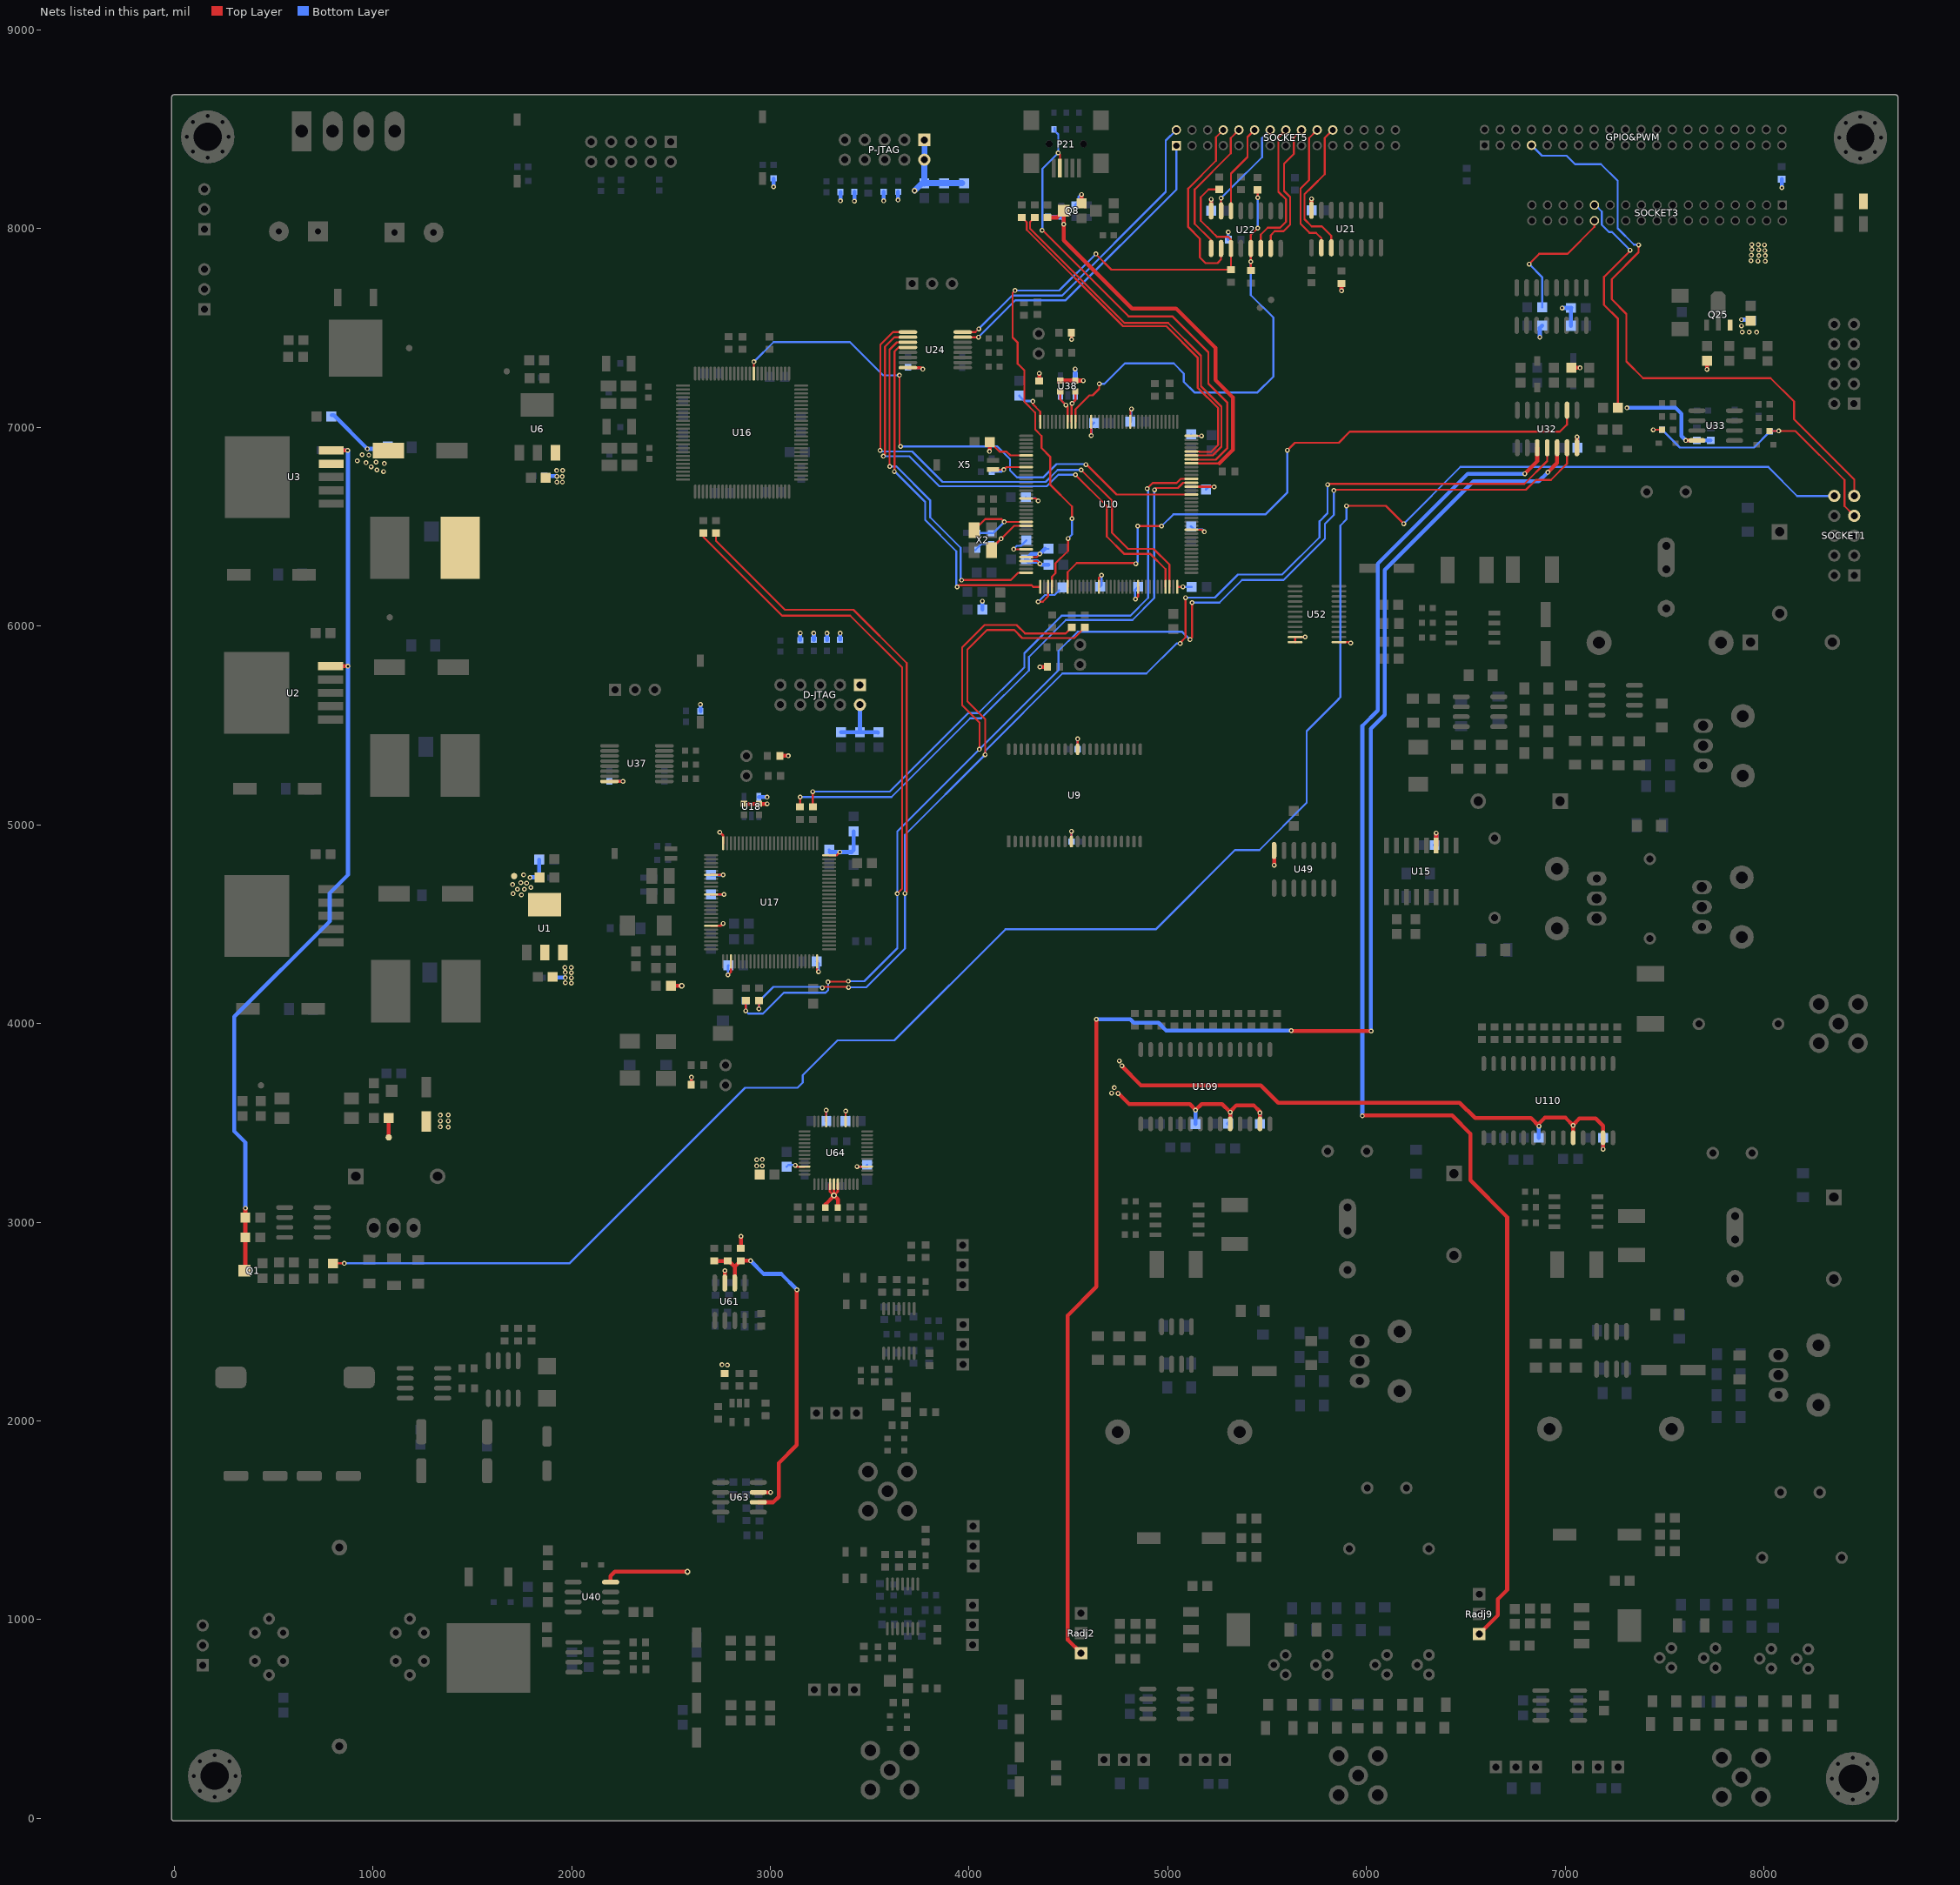
[diagram p0: the nets of this part, all layers, seen from the top]
# Altium PCB MISC82309.PcbDoc (part 12 of 14)
Units mil, origin at the board's own origin, x right, y up, seen from the top; angles counter-clockwise.
Board outline 8687.03 x 8687.86 mil, 4 copper layers (Top Layer, GND, POWER, Bottom Layer); 747 components, 583 nets, 2530 pads, 1834 vias.

## Via types
v1: diameter 24, hole 12, Top Layer to Bottom Layer, 1799 vias
v2: diameter 30, hole 15, Top Layer to Bottom Layer, 26 vias
v3: diameter 40, hole 20, Top Layer to Bottom Layer, 9 vias

## Nets (pads, with @x,y where several pads share a name; then routed paths per layer and width w, separated by ;. In a path a pad name is that pad's centre, name@x,y a point inside that pad or via, vN(x,y) a via of type N, cw(c..) or ccw(c..) an arc to the next point about the centre after c; other vN are vias at no path point) (continued)
P_OSC32_OUT: C99.2 U10.9 X5.4 | length 237.1
  Top Layer w10: X5.4@4121,6787.38 v1@4175.38,6787.38 ; v1(4175,6787) v1@4175.38,6787.38 ; U10.9@4287.65,6800.01 4189.01,6800.01 4176.38,6787.38 v1@4175.38,6787.38
  Bottom Layer w10: C99.2@4114.5,6777 4165,6777 v1(4175,6787)
P_OSC_IN: C40.2 R66.1 U10.23 X2.1 | length 459.3
  Top Layer w10: X2.1@4026,6483 4081,6538 4164,6538 v1(4177.58,6524.42) U10.23@4287.65,6524.42
  Bottom Layer w10: C40.2@4032.5,6469 4109.5,6469 R66.1@4111,6467.5 4120.67,6467.5 v1(4177.58,6524.42)
P_OSC_OUT: C41.2 R66.2 U10.24 X2.3 | length 381.6
  Top Layer w10: X2.3@4112.61,6383 4112.61,6390.61 4226.73,6504.73 U10.24@4287.65,6504.73
  Bottom Layer w10: C41.2@4032.5,6383 4062,6412.5 R66.2@4111,6412.5 4134.5,6412.5 v1(4161,6439)
P_RS232_RXD: SOCKET5.2 U24.8 | length 1648.1
  Top Layer w10: U24.8@3967.8,7479.57 4032.57,7479.57 v1(4049,7496)
  Bottom Layer w10: v1(4049,7496) 4217,7664 4469,7664 4990,8185 4990,8443.74 SOCKET5.2@5043,8496.74
P_RS232_TXD: SOCKET5.1 U24.7 | length 1604
  Top Layer w10: U24.7@3967.8,7453.98 v1(4048,7454)
  Bottom Layer w10: v1(4048,7454) 4234,7640 4486,7640 5043,8197 SOCKET5.1@5043,8418
P_SCL: R208.2 U10.136 U38.1 | length 206.2
  Top Layer w10: U10.136@4515.99,7028.35 4515.99,7069 4515.99,7117.99 v1(4519,7121) 4535,7137 R208.2@4535,7180.5
  Bottom Layer w10: v1(4519,7121) 4534.4,7136.4 U38.1@4534.4,7160.76
P_SDA: R209.2 U10.137 U38.3 | length 227.2
  Top Layer w10: R209.2@4459,7180.5 4459,7141 4487,7113 v1(4487.35,7112.65) 4496.31,7103.69 4496.31,7089 U10.137@4496.31,7028.35
  Bottom Layer w10: U38.3@4459.6,7160.76 4459.6,7140.4 v1(4487.35,7112.65)
P_USART2_RX: U10.37 U24.12 | length 1814.6
  Top Layer w10: v1@3625,6779 3625,7382 3645.8,7402.8 U24.12@3692.2,7402.8 ; v1@3940,6198 3947.5,6205.5 4314.5,6205.5 4322.35,6197.65 U10.37@4358.51,6197.65
  Bottom Layer w10: v1@3626,6778 3779,6625 3779,6534 3936,6377 3936,6204 v1@3942,6198
  other v1: 3940,6197 3624,6778
P_USART2_TX: U10.36 U24.11 | length 1774.7
  Top Layer w10: v1@3600,6804 3600,7391 3637.39,7428.39 U24.11@3692.2,7428.39 ; v1@3963,6232 4210,6232 4246.51,6268.51 U10.36@4287.65,6268.51
  Bottom Layer w10: v1(3601,6803) 3635,6803 3806,6632 ; 3805,6631 3805,6547 3958,6394 3958,6237 v1@3963,6232
  other v1: 3963,6231
P_USART3_RX: U10.70 U24.9 | length 2647.5
  Top Layer w10: v1@3554,6884 3554,7416 3617.57,7479.57 U24.9@3692.2,7479.57 ; v1(4564,6786) 4719,6631 4719,6470 4800,6389 4929,6389 5008.12,6309.88 U10.70@5008.12,6197.65
  Bottom Layer w10: v1(3552,6884) 3558,6878 3558.06,6878 3559.06,6879 3714,6879 3867,6726 4386,6726 4446,6786 v1(4564,6786)
P_USART3_TX: U10.69 U24.10 | length 2577.3
  Top Layer w10: v1(3569,6855) 3577,6863 3577,7406 3624.98,7453.98 U24.10@3692.2,7453.98 ; v1@4535,6756 v1(4535,6762) 4693,6604 4693,6450.72 4779.72,6364 4911.43,6364 4988.43,6287 U10.69@4988.43,6197.65
  Bottom Layer w10: v1(3569,6855) 3699,6855 3850,6704 4391,6704 4449,6762 v1(4535,6762)
P_VDDA: C37.2 C38.2 R276.2 U10.32 U10.33 | length 452.8
  Top Layer w10: U10.33@4287.65,6327.57 4343.43,6327.57 v1(4357,6314) ; U10.32@4287.65,6347.25 4340.25,6347.25 v1(4356,6363)
  Bottom Layer w10: v1(4356,6363) 4382,6389 C37.2@4399.5,6389 ; C38.2@4394.5,6314 C38.2@4399.5,6309
  Bottom Layer w20: C37.2@4382,6389 v1(4356,6363) 4313.5,6363 R276.2@4286.5,6336 4297.5,6325 4346,6325 v1(4357,6314) 4362,6309 C38.2@4399.5,6309
POWER-ON/OFF: GPIO&PWM.7 SOCKET1.9 | length 3090.6
  Top Layer w10: v1@7364,7918 v1(7369,7918) ; v1@7369,7916 7369,7881 7234,7746 7234,7645 7308,7571 7308,7332 7392,7248 8033,7248 8151,7130 8151,7041 8454,6738 SOCKET1.9@8454,6655
  Bottom Layer w10: GPIO&PWM.7@6830.22,8420 6883.22,8367 7007,8367 7049,8325 7180,8325 7264,8241 7264,8002 7346,7920 ; 7346,7919 v1@7366,7919 ; v1@7364,7918 v1(7369,7918)
POWER_CONTROL: R8.1 SOCKET1.10 | length 10132.2
  Top Layer w10: R8.1@799.5,2793 v1(856,2793) ; v1(5899,6605) 6097,6605 v1(6187,6515)
  Bottom Layer w10: v1(856,2793) 1989,2793 2873,3677 3137,3677 3163,3703 3163,3740 3338,3915 3624,3915 4183,4474 4939,4474 5338,4873 5461,4873 5699,5111 5699,5472 5860.5,5633.5 ; 5860,5634 5868,5642 5868,6506 5899,6537 v1(5899,6605) ; v1@6189,6517 6473,6801 8022,6801 ; 8022,6800 8167,6655 SOCKET1.10@8354,6655 SOCKET1.10@8349.5,6659.5
POWER_ENABLE: Q1.3 R7.1 R399.2 R555.2 U2.5 U3.5 | length 4637.2
  Top Layer w20: Q1.3@354,2756 358.5,2760.5 R399.2@358.5,2924 R7.1@358.5,3024 v1(358.5,3070.5) ; U2.5@787.22,5797.86 v1(874.86,5797.86) ; U3.5@790.22,6883.86 v1(872.86,6883.86)
  Bottom Layer w20: v1(358.5,3070.5) 358.5,3402.5 303,3458 303,4034 783,4514 783,4656 875,4748 875,6882 v1@873,6884 ; R555.2@797,6885 798.14,6883.86 v1(872.86,6883.86)
PRE-CH_A: R345.2 R349.2 R515.2 R565.1 U32.13 | length 9740.3
  Top Layer w10: R345.2@2663,6468.5 2663,6449 3059,6053 3402,6053 3663,5792 3663,4678 v1@3638.5,4653.5 ; v1@2877,4065 R515.2@2877,4115.5 ; v1@3292,4211 v1@3390,4211 ; v1(4052,5380) 4053,5381 4053,5514 3965,5602 3965,5893 4078,6006 4239,6006 4282.21,5962.79 4486.28,5962.79 R349.2@4517,5993.5 ; 5122,5942 v1(5122,6118) ; v1(5836,6682) 5840,6686 6802,6686 6852,6736 6928,6736 7009,6817 U32.13@7009,6897.51
  Bottom Layer w10: v1(2876,4064) 2890,4050 2963,4050 3068,4155 3278,4155 3291,4168 v1@3291,4208 ; v1@2876,4067 R565.1@2876,4115.5 ; v1(3392,4213) 3473,4213 3639,4379 v1(3639,4653) 3639,4967 v1(4052,5380) 4450,5778 4450,5875 4546,5971 5073,5971 v1(5112,5932) ; v1(5122,6118) 5260,6118 5374,6232 5583,6232 5791,6440 5791,6514 5836,6559 v1(5836,6682)
  other v1: 3290,4209
PRE-CH_B: R346.2 R348.2 R516.2 R564.1 U32.11 | length 9489.9
  Top Layer w10: R346.2@2727,6468.5 2727,6429 3074,6082 3418,6082 3686,5814 v1@3686,4663 ; v1@2943,4067 R516.2@2943,4115.5 ; v1@3267,4185 v1@3394,4185 ; v1(4081,5353) 4081,5532 3992,5621 3992,5882 4090,5980 4228,5980 4268,5940 4529.5,5940 R348.2@4583,5993.5 ; v1@5062,5915.94 5089,5942.94 v1(5089,6143) ; v1(5804,6712) 5808,6716 6794,6716 6909,6831 U32.11@6909,6897.51
  Bottom Layer w10: v1@2940,4071 v1@2940,4072 ; v1@2943,4070 2943,4112 3016,4185 v1@3257,4185 ; v1(2943,4074) 2943,4067 v1@2944.5,4068.5 ; v1(3394,4182) 3483,4182 3678,4377 v1(3678,4655) 3678,4950 v1(4081,5353) 4081,5372 4470,5761 4892,5761 5044,5913 v1(5062,5913) ; v1(5089,6143) 5237,6143 5353,6259 5575,6259 5763,6447 5763,6527 5804,6568 v1(5804,6712) 5806,6710 v1@5806,6712
  other v1: 3262,4180
PRE-CHARGE_A: Radj2.1 U32.12 | length 8198
  Top Layer w20: Radj2.1@4564,832 4497,899 4497,2531 4641,2675 v1(4641,4022) ; v1(5621,3965) 5624,3962 v1(6023,3962) ; v1(6912,6774) 6959,6821 U32.12@6959,6897.51
  Bottom Layer w20: v1(4641,4022) 4811,4022 4829,4004 4953,4004 4992,3965 v1(5621,3965) ; v1@6021,3965 6022,3966 6022,5484 6091,5553 6091,6282 6538,6729 6867,6729 v1(6912,6774)
PRE-CHARGE_B: Radj9.1 U32.10 | length 7127.3
  Top Layer w20: v1@5980,3537 6431,3537 6523,3445 6523,3211 6708,3026 6708,1150 6661,1103 6661,1022 Radj9.1@6567,928 ; v1(6797,6767) 6859,6829 U32.10@6859,6897.51
  Bottom Layer w20: v1(5979,3536) 5979,5498 6057,5576 6057,6314 6510,6767 v1(6797,6767)
PRINT-RST: U10.93 U16.85 | length 2907.2
  Top Layer w10: U16.85@2917.06,7271.24 v1(2917.06,7329.94) ; v1@3650,6910 v1(3650,7262) ; v1(4588,6813) 4591,6813 4742,6662 5118.14,6662 U10.93@5118.35,6662.21
  Bottom Layer w10: v1(2917.06,7329.94) 3016.11,7429 3401,7429 3568,7262 v1(3650,7262) ; v1(3656,6904) 4143,6904 4206,6841 4206,6784 4242,6748 4373,6748 4440.38,6815.38 4585.62,6815.38 v1(4588,6813) v1@4589,6812
PRODUCT-S: U10.44 U32.2 | length 3194.3
  Top Layer w10: U10.44@4496.31,6197.65 4496.31,6271.31 4542,6317 v1@4836,6317 ; v1(4848,6503) v1(4969,6503) ; v1(5602,6885) 5639.91,6922.91 5860.91,6922.91 5916,6978 6973,6978 7009,7014 U32.2@7009,7086.49
  Bottom Layer w10: v1(4839,6314) 4848,6323 v1(4848,6503) ; v1(4969,6503) 5028,6562 5491,6562 5602,6673 v1(5602,6885)
PRODUCT_SENSOR_: R493.1 SOCKET3.25 | length 1192.5
  Top Layer w10: R493.1@7265.5,7098 7265.5,7546.5 7195,7617 7195,7757 7326,7888 v1(7326,7892)
  Bottom Layer w10: SOCKET3.25@7147.12,8119 SOCKET3.25@7153.06,8113.06 ; SOCKET3.25@7155,8115 7184,8086 7184,8019 7220,7983 7235,7983 v1(7326,7892) v1@7326,7888
REFINA: C506.1 C507.1 U64.5 U64.6 U64.7 | length 330.6
  Top Layer w12: U64.5@3300.47,3191.52 3300.47,3154.53 v2(3320,3135) ; U64.6@3320.16,3191.52 3320.16,3135.16 3339.84,3154.84 U64.7@3339.84,3191.52
  Top Layer w20: C506.1@3277,3075.95 3277,3077.5 C506.1@3278,3078.5 ; C506.1@3278,3076 C506.1@3278,3078.5 ; C507.1@3340,3077.5 3340,3115 3320.16,3134.84 3320.08,3134.92 v2(3320,3135) 3320,3132.41 3278,3090.41 C506.1@3278,3078.5
SENSOR_DECTET: R155.1 SOCKET3.26 | length 681.9
  Top Layer w10: v1(6818,7822) 6869,7873 7011,7873 7147.12,8009.12 SOCKET3.26@7147.12,8040.26
  Bottom Layer w10: v1(6818,7822) 6883.5,7756.5 R155.1@6883.5,7605
SENSOR_DRV: C163.2 C363.2 R175.1 R375.1 SOCKET1.7 | length 1426.9
  Top Layer w10: v1(7443,6988) R175.1@7487.5,6988 ; R375.1@8027.5,6982 v1(8074,6982) 8158,6982 8405,6735 8405,6604 SOCKET1.7@8454,6555
  Bottom Layer w10: v1(7443,6988) C163.2@7487.5,6988 7576.5,6899 7949.5,6899 C363.2@8029.5,6979 8032.5,6982 v1(8074,6982)
SPI2_CS: R101.1 R405.2 U10.40 U22.3 | length 3442.1
  Top Layer w10: v1(4231,7689) 4219,7677 4219,7452 4245,7426 4245,7320 4278,7287 4278,7264 4278,7129 4332,7075 ; 4333,7075 4333,6989 4365,6957 4365,6896 4408,6853 4408,6712 4518,6602 v1(4518,6541) ; U10.40@4417.57,6197.65 4417.57,6248.57 4435,6266 4435,6316 4498,6379 v1(4498,6441) ; v1@4636,7874 4716.5,7793.5 R405.2@5313.5,7793.5 ; 5224,7981 5225,7981 5246.5,7959.5 5303.5,7959.5 5318,7945 U22.3@5318,7900.51 5318,7794 R405.2@5319,7793 ; 5224.5,7981.5 5166,8040 5166,8158 5205.5,8197.5 R101.1@5258,8197.5 R101.1@5269,8197.5 ; R405.2@5314,7794 R405.2@5313.5,7793.5 ; R405.2@5318,7793.5 R405.2@5313.5,7793.5
  Bottom Layer w10: v1(4231,7689) 4454,7689 v1(4638,7873) ; v1(4498,6441) 4518,6461 v1(4518,6541)
SPI2_CS_N: SOCKET5.10 U22.1 | length 723
  Top Layer w10: U22.1@5218,7900.51 5218,7942 5135,8025 5135,8197 5317,8379 5317,8455.78 SOCKET5.10@5357.96,8496.74
SPI2_CS_P: SOCKET5.8 U22.2 | length 919.7
  Top Layer w10: U22.2@5268,7900.51 5268,7845 5250,7827 5190,7827 5162,7855 5162,7949 5103,8008 5103,8202 5243,8342 5243,8460.52 SOCKET5.8@5279.22,8496.74
SPI2_MISO_N: SOCKET5.22 U21.3 | length 738.3
  Top Layer w10: 5725,8210 5688,8173 5688,8048 5724,8012 5775,8012 5823,7964 U21.3@5823,7903.51 ; 5725.5,8209.5 5790,8274 5790,8456.34 SOCKET5.22@5830.4,8496.74
SPI2_MISO_P: SOCKET5.20 U21.2 | length 689.7
  Top Layer w10: 5713,7979 5746,7979 5773,7952 U21.2@5773,7903.51 ; 5713,7980 5668,8025 5668,8202 5711,8245 5711,8456.08 SOCKET5.20@5751.66,8496.74
SPI2_MOSI: R103.1 R408.2 U10.135 U22.5 | length 2336.5
  Top Layer w10: U10.135@4535.68,7028.35 4535.68,7090.68 4606,7161 4622,7161 4655,7194 v1(4655,7219) ; v1@5417,7836 5418,7835 R408.2@5418,7789.5 ; v1(5418,7834) U22.5@5418,7900.51 5418,7968 v1(5453,8003) ; R103.1@5448,8194.5 5453,8189.5 v1(5453,8156)
  Bottom Layer w10: v1(4655,7219) 4681,7219 4784,7322 5030,7322 5081,7271 5081,7229 5134,7176 5452,7176 5532,7256 5532,7552 5418,7666 v1(5418,7834) ; v1(5453,8003) v1(5453,8156)
SPI2_MOSI_N: SOCKET5.18 U22.7 | length 712.4
  Top Layer w10: U22.7@5518,7900.51 5518,7967 5538,7987 5583,7987 5616,8020 5616,8159 5585,8190 5585,8327 5634,8376 5634,8457.82 SOCKET5.18@5672.92,8496.74
SPI2_MOSI_P: SOCKET5.16 U22.6 | length 716.3
  Top Layer w10: U22.6@5468,7900.51 5468,7970 5503,8005 5565,8005 5595,8035 5595,8148 5557,8186 5557,8459.56 SOCKET5.16@5594.18,8496.74
SPI2_SCK_N: SOCKET5.14 U22.15 | length 509.7
  Top Layer w10: U22.15@5268,8089.49 v1(5268,8154)
  Bottom Layer w10: v1(5268,8154) 5321.5,8207.5 5474,8360 5474,8455.3 SOCKET5.14@5515.44,8496.74
SPI2_SCK_P: SOCKET5.12 U22.14 | length 456.4
  Top Layer w10: U22.14@5318,8089.49 5318,8278 5401.08,8361.08 5401.08,8461.12 SOCKET5.12@5436.7,8496.74
USART6_RX: R513.2 U10.97 | length 3003.2
  Top Layer w10: R513.2@3214,5090.5 v1(3214,5167) ; v1(4896,6692) 4924,6720 5044,6720 5064.95,6740.95 U10.97@5118.35,6740.95
  Bottom Layer w10: v1(3214,5167) 3601,5167 3996,5562 4048,5562 4278,5792 4278,5863 4466,6051 ; 4466,6052 4811,6052 4901,6142 4901,6687 v1(4896,6692)
USART6_TX: R514.2 U10.96 | length 3031.3
  Top Layer w10: R514.2@3150,5090.5 v1(3150,5140) ; v1(4933,6686) 4942,6695 5051,6695 5077.27,6721.27 U10.96@5118.35,6721.27
  Bottom Layer w10: v1(3150,5140) 3610,5140 4006,5536 4060,5536 4301,5777 4301,5845 4487,6031 4822,6031 4932,6141 4932,6685 v1(4933,6686)
USBDM: R95.2 U10.103 | length 1860.3
  Top Layer w10: R95.2@4330,8056.5 4307,8033.5 4307,8001.04 4782.04,7526 5001.41,7526 5167,7360.41 5167,7207.63 5270,7104.63 5270,6902.96 5226.1,6859.06 U10.103@5118.35,6859.06
USBDP: R96.2 U10.104 | length 1832.1
  Top Layer w10: R96.2@4266,8056.5 4290,8032.5 4290,7994 4775,7509 4994.37,7509 4994.37,7507.59 5150,7351.96 5150,7200.59 5253,7097.59 5253,6911.41 5218.49,6876.91 5160.84,6876.91 5159,6878.75 U10.104@5118.35,6878.75
USBID: ESD23.1 P21.4 U10.102 | length 2454.3
  Top Layer w10: v1(4368,7992) 4370,7992 4803,7559 5023,7559 5204,7378 5204,7220 5300,7124 5300,6896 5241.6,6837.6 5120.13,6837.6 U10.102@5118.35,6839.38 ; v1(4449,8381) 4457.5,8372.5 P21.4@4457.5,8304.95
  Bottom Layer w10: v1(4368,7992) 4369.25,7993.25 4369.25,8301.25 v1(4449,8381) 4449,8474 4430,8493 ESD23.1@4430,8506.68
VBUS: C240.2 C241.2 Q8.3 R57.2 U10.101 | length 2124.5
  Top Layer w11: U10.101@5118.35,6819.69 5260.69,6819.69
  Top Layer w20: R57.2@4394,8056.5 4442.5,8056.5 Q8.3@4476,8090 4476,7942 4820,7598 5042,7598 5240,7400 5240,7238 5327,7151 5327,6886 5260.69,6819.69
  Bottom Layer w20: C241.2@4397,8060.5 C240.2@4460.5,8060.5 ; C240.2@4465,8060.5 4477,8048.5 v1(4477,8023)
VCC: C1.2 C6.2 C10.1 C15.1 C17.1 C18.2 C19.2 C56.1 C82.2 C83.2 C151.2 C154.2 C210.2 C370.2 FB18.2 FB25.1 L3.2 Q8.2 R3.1 R5.1 R35.2 R36.2 R150.2 R156.2 R165.2 R479.2 TP3.1 U1.3 U3.4 U6.3 U15.11 U21.16 U22.16 U32.14 U33.8 U40.8 U49.14 U52.1 U61.3 U63.3 | length 2740
  Top Layer w12: U52.1@5861.24,5919.25 5915.75,5919.25 v1(5920,5915)
  Top Layer w20: TP3.1@1080,3427 R5.1@1080,3511 ; U40.8@2196.49,1189 2196.49,1219.49 2218,1241 v2(2583,1241) ; U61.3@2771,2694.49 v1(2771,2756) ; U63.3@2939.49,1641 v1(3001,1641) ; Q8.2@4566,8127 v1(4566,8172) ; U22.16@5218,8089.49 v1(5218,8148) ; v1(5535,4797) U49.14@5535,4870.49 ; U21.16@5723,8092.49 v1(5723,8150) ; v1(5874,7688) R35.2@5874,7724.5 ; U15.11@6351,4896 v1(6351,4959) ; R165.2@7030,7299.5 v1(7074.5,7299.5) ; U32.14@7059,6874 v1(7059,6952) ; v1(7606,6934) U33.8@7662.51,6934
  Bottom Layer w15: R150.2@4535,8119.5 4552,8136.5 4552,8159 v1@4562,8169 ; R36.2@5304.5,7945 v1(5304.5,7983.5)
  Bottom Layer w20: R3.1@793,7061 803,7061 v1@971,6893 ; v1@968,6893 v1@971,6893 ; v1@972,6893 v1@971,6893 ; C15.1@1075,6890 1073,6892 v1(972,6892) v1@971,6893 ; C19.2@1863.5,6755 v1@1925,6755 ; C6.2@1922.5,4231 1965,4231 v1@1966,4232 ; C82.2@5218.5,8090 v1@5218.5,8145.5 ; C83.2@5723,8104 v1(5723,8150) ; C56.1@6342.5,4898 6351,4906.49 v1@6351,4958 ; v1(6872,7454) 6872,7500.5 R156.2@6883.5,7512 ; v1(6984,7601) C151.2@7028.5,7601 ; FB18.2@7028.61,7511 7028.61,7601.61 C151.2@7030,7603 ; C154.2@7059,6895.51 C154.2@7060.5,6897 v1@7060.5,6950.5 ; v1(7310,7098) 7555.04,7098 7584,7069.04 7584,6956 v1(7606,6934) ; v1@7610.5,6934.5 C370.2@7663,6934.5 C210.2@7732,6934.5
  other v1: 2784,2282 2757,2283 1379,3479 1339,3480 1340,3510 1380,3510 1339,3539 1380,3540 1999,4203 1969,4205 1999,4230 1968,4231 1999,4256 1968,4257 1967,4282 1998,4282 1954,6724 1926,6725 1953,6753 1926,6754 1054,6778 1925,6783 1955,6784 1021,6786 991,6802 1058,6818 966,6822 1016,6825 921,6832 980,6860 946,6862 8006,7836 7970,7837 7935,7839 8006,7864 7974,7865 7936,7867 8004,7890 7973,7894 7938,7895 8003,7918 7938,7920 7971,7920
VDD_3V3: C2.2 C7.2 C30.1 C31.1 C86.2 C87.2 C88.2 C90.2 C123.2 C124.2 C125.2 C126.2 C127.2 C128.2 C129.2 C130.2 C131.2 C132.2 C133.2 C134.2 C141.2 C142.2 C143.2 C146.2 C147.2 C148.2 C181.2 C220.2 C242.2 C243.2 C245.2 C246.2 C247.2 C248.2 C249.2 C250.2 C251.2 C252.2 C253.2 C254.2 C255.2 C282.1 C283.1 D-JTAG.1 D-JTAG.2 L21.2 P-JTAG.1 P-JTAG.2 Q25.3 R1.1 R63.1 R111.1 R112.1 R113.1 R208.1 R209.1 R235.1 R270.2 R271.2 R272.2 R273.2 R274.2 R277.1 R283.2 R404.1 R587.2 R588.2 R589.2 R590.2 R592.2 R593.2 R594.2 R596.1 R598.2 TP1.1 U1.2 U1.4 U9.11 U9.33 U10.6 U10.17 U10.30 U10.39 U10.52 U10.62 U10.72 U10.84 U10.95 U10.108 U10.121 U10.131 U10.144 U17.6 U17.11 U17.19 U17.28 U17.50 U17.75 U17.100 U18.5 U24.16 U37.16 U38.5 U52.23 U52.24 U64.15 U64.28 U64.33 U64.46 U109.24 U109.27 U110.24 U110.27 | length 9934.1
  Top Layer w10: v1(2787,4245) v1@2788.5,4246.5 ; v1@2789,4246 2802.15,4259.15 U17.28@2802.15,4312.76 ; v1(3125,3287) 3131.9,3280.1 U64.46@3172.52,3280.1 ; U17.50@3235.22,4312.76 3235.22,4268.78 v1(3243,4261) ; U64.33@3280.79,3506.48 v1(3280.79,3563.79) ; U64.28@3379.21,3506.48 v1(3379.21,3560.21) ; v1(3436.1,3280.1) U64.15@3487.48,3280.1 ; v1(4103,6879) v1@4103,6881 ; C128.2@4103,6925.5 C128.2@4103.5,6926 ; C128.2@4122,6910 4154,6878 4189,6878 4207.94,6859.06 U10.6@4287.65,6859.06 ; v1(4224.38,6386.62) U10.30@4287.65,6386.62 ; U10.17@4287.65,6642.53 4335.47,6642.53 v1(4348,6630) ; v1@4322,7132 v1(4321,7131) 4321,7117 4358.51,7079.49 U10.144@4358.51,7028.35 ; v1(4348,6123) 4371,6123 4397.88,6149.88 U10.39@4397.88,6197.65 ; U9.11@4514.96,4916 v1(4514.96,4967.96) ; U9.33@4546.46,5380.57 v1(4546.46,5432.46) ; U10.131@4614.42,7028.35 4614.42,6959.58 v1(4615,6959) ; U10.52@4653.79,6197.65 4653.79,6242.79 v1(4667,6256) ; U10.121@4811.27,7028.35 4812,7029.09 4812,7090 4810,7092 4811,7093 v1(4817,7093) ; v1(4838,6136) 4850.64,6148.64 U10.62@4850.64,6197.65 ; U10.72@5047.49,6197.65 v1(5075.65,6197.65) ; U10.84@5118.35,6485.05 5172.95,6485.05 v1(5184,6474) ; U10.108@5118.35,6957.49 v1(5169.51,6957.49)
  Top Layer w12: U17.19@2701.76,4491.89 2750.89,4491.89 v1(2763,4504) ; U17.11@2701.76,4649.37 v1(2767.63,4649.37) ; U17.6@2701.76,4747.8 v1(2762.8,4747.8) ; v1(2746,4963) 2762.78,4946.22 U17.100@2762.78,4907.24 ; U17.75@3296.24,4846.22 3333.22,4846.22 v1(3350,4863) ; U10.95@5118.35,6701.58 v1@5230.58,6701.58 ; v1@5231,6702 v1@5230.58,6701.58 ; v1(5233,6701) 5232,6701 5231.42,6701.58 v1@5230.58,6701.58 ; U52.24@5640.76,5919.25 5641,5919.49 U52.23@5641,5943 ; U52.23@5640.76,5944.84 v1(5690.84,5944.84)
  Top Layer w15: U37.16@2191.2,5218.43 v1(2258.43,5218.43) ; R272.2@2602.5,3691 v1(2602.5,3729.5)
  Top Layer w16: U24.16@3692.2,7300.43 v1@3758.57,7300.43 ; v1(4515.5,7442.5) R271.2@4515.5,7476
  Top Layer w20: R235.1@2499.5,4190 v2(2554,4190) ; R598.2@2852,2869.5 2852,2923 v1(2852,2929) ; R112.1@2868,5105.5 R111.1@2939.5,5105.5 ; R111.1@2943,5105.5 v1(2984.5,5105.5) ; R273.2@3048.5,5347 v1(3090,5347) ; C128.2@4103.5,6926 4103.5,6881.5 v1@4104,6881 ; R274.2@4353,7234 v1(4353,7272) ; v1(4357,5794) 4362,5794 4363,5795 R270.2@4393.5,5795 ; R209.1@4459,7235.5 v1(4575.5,7235.5) ; v1@4749,3651 4806,3594 5111,3594 5140,3565 5170,3595 5273,3595 v1(5314,3554) U109.24@5314,3494.99 ; v1@4767,3787 4865,3689 5468,3689 5555,3602 6469,3602 6547,3524 6828,3524 v1@6867,3485 ; v1@5315,3558 5346,3589 5432,3589 5464,3557 v1(5464,3550) U109.27@5464,3494.99 ; v1(6868,3484) v1@6867,3485 ; U110.24@7040,3424.99 v1(7040,3487) 7001,3526 6898,3526 6867,3495 v1@6867,3485 ; v1@7041,3492 7071,3522 7153,3522 7190,3485 U110.27@7190,3424.99 v1(7190,3368) ; v1(7713,7292) R283.2@7713,7335.5
  Bottom Layer w10: C86.2@3082,3279.5 3090.5,3288 v1@3122,3288 ; C252.2@3233.5,4313 3244,4302.5 v1@3244,4266 ; C254.2@3282.5,3509 v1@3282.5,3561.5 ; C243.2@3378.5,3509 v1@3378.5,3556.5 ; v1@3437,3280 3478.5,3280 C250.2@3488,3289.5 ; v1@4226,6390 4240,6404 4260.5,6404 C130.2@4289,6432.5 ; C129.2@4285.5,6649 4290.5,6644 4333,6644 v1@4345,6632 ; v1(4348,6123) 4382,6157 4431,6157 C143.2@4453,6179 ; v1@4515,4965 v1@4515.5,4964.5 ; v1(4546.46,5432.46) 4546.5,5432.41 C148.2@4546.5,5381 ; C142.2@4660.5,6198 4667,6204.5 v1(4667,6256) v1@4667,6258 ; C125.2@4811.5,7028 4817,7033.5 v1@4817,7089 ; v1@4835,6140 4835,6182.5 C134.2@4850.5,6198 ; v1(5075.65,6197.65) 5076.29,6197 C141.2@5120.5,6197 ; C124.2@5118,6964.5 5126.5,6956 v1@5170,6956
  Bottom Layer w12: C245.2@2701,4649.5 2760.5,4649.5 v1@2761,4649 ; C87.2@2701,4747.5 2759.5,4747.5 v1@2760,4748 ; v1@2788,4247 2787,4246 2787,4290.5 C251.2@2789.5,4293 ; C247.2@3296,4875.5 C247.2@3308.5,4863 ; C127.2@4253,7159.5 4279.5,7133 v1@4321,7133 ; C147.2@4515.5,4915 v1@4515.5,4964.5 ; v1@4615,6961 4615,7009.5 C126.2@4628.5,7023 ; C123.2@5117,6501.5 5132.5,6486 5174,6486 v1@5183,6477 ; C146.2@5192.5,6688 5205.5,6701 v1@5232,6701
  Bottom Layer w15: C181.2@2191,5218.5 v1@2254.5,5218.5
  Bottom Layer w16: C90.2@3693,7302.5 3695.5,7300 3758,7300 v1@3764,7294
  Bottom Layer w20: v1@1794,4736 1834,4736 1837.5,4739.5 R1.1@1837.5,4825 ; R113.1@2648,5571.5 v1(2648,5606) ; U18.5@2942.4,5139.24 v1(2983.24,5139.24) ; v1(3016.5,8210.5) R63.1@3016.5,8253 ; R594.2@3151,5929.5 v1(3151,5965) ; R593.2@3219,5930.5 v1(3219,5964) ; R596.1@3285,5930.5 v1(3285,5964) ; C247.2@3300,4863 3308.5,4863 v1(3350,4863) 3409.5,4863 C253.2@3420,4873.5 ; R592.2@3351,5931.5 v1(3351,5964) ; v1(3353,8140) R588.2@3353,8184.5 ; C249.2@3356,5465.5 3448.5,5465.5 C255.2@3451,5468 ; C253.2@3419,4878 C88.2@3419,4967.5 ; v1(3423,8139) R590.2@3423,8185.5 ; D-JTAG.2@3451,5593 C255.2@3451,5468 ; C242.2@3541,5464 3539.5,5465.5 C255.2@3451,5465.5 C255.2@3451,5468 ; v1(3570,8140) R587.2@3570,8185.5 ; v1(3643,8144) R589.2@3643,8185.5 ; R277.1@4067.5,6083 v1(4067.5,6125.5) ; U38.5@4534.4,7255.24 v1(4534.4,7294.4) ; C30.1@5139.5,3494 v1(5139.5,3563.5) ; C246.2@5303.5,3496 5314,3506.5 v1@5314,3551 ; C31.1@5463.5,3495 v1@5463.5,3549.5 ; C282.1@6866.5,3425 6866.5,3482.5 v1(6868,3484) ; C283.1@7187,3420 7190,3417 v1(7190,3368) ; v1@7888,7542 7930.5,7542 C248.2@7935,7537.5 ; v1(8090,8206) R404.1@8090,8249.5
  Bottom Layer w30: v2(3726,8191) 3763.5,8228.5 C131.2@3775,8228.5 ; C131.2@3771,8231 3775,8227 3775,8333 3776,8334 3776,8430 P-JTAG.1@3780,8434 ; C131.2@3776,8230 C133.2@3966,8230
  other v1: 2931,3283 2960,3284 2932,3315 2960,3316 4750,3648 4717,3650 4731,3677 4769,3787 4756,3812 1748,4647 1705,4653 1728,4676 1763,4676 1795,4685 1703,4699 1774,4707 1744,4709 1791,4735 1759,4748 3767,7293 7963,7479 7890,7480 7925,7480 7886,7511 7886,7542
VOCM: C599.1 R598.1 R599.2 U61.2 U63.2 | length 1769.4
  Top Layer w20: C599.1@2725,2805 2791,2805 2821,2775 U61.2@2821,2694.49 ; 2822,2777 2851.5,2806.5 R598.1@2852,2806.5 2900.5,2806.5 v1(2901,2806) ; U63.2@2939.49,1591 3015,1591 3043,1619 3043,1788 3133,1878 3133,2659 v1(3134,2660)
  Bottom Layer w20: v1(2901,2806) 2967,2740 3055,2740 v1@3134.5,2660.5 ; v1(3134,2660) v1@3134.5,2660.5 ; v1@3135,2660 v1@3134.5,2660.5
pads on no net: CPLD-JTAG.6 CPLD-JTAG.7 CPLD-JTAG.8 GPIO&PWM.6 GPIO&PWM.8 GPIO&PWM.9 GPIO&PWM.16 GPIO&PWM.25 GPIO&PWM.26 GPIO&PWM.27 GPIO&PWM.28 GPIO&PWM.34 GPIO&PWM.35 P21.10 P21.11 PCB_MH1.0 PCB_MH1.1 PCB_MH1.2 PCB_MH1.3 PCB_MH1.4 PCB_MH1.5 PCB_MH1.6 PCB_MH1.7 PCB_MH1.8 PCB_MH1.9 PCB_MH1.10 PCB_MH2.0 PCB_MH2.1 PCB_MH2.2 PCB_MH2.3 PCB_MH2.4 PCB_MH2.5 PCB_MH2.6 PCB_MH2.7 PCB_MH2.8 PCB_MH2.9 PCB_MH2.10 PCB_MH3.0 PCB_MH3.1 PCB_MH3.2 PCB_MH3.3 PCB_MH3.4 PCB_MH3.5 PCB_MH3.6 PCB_MH3.7 PCB_MH3.8 PCB_MH3.9 PCB_MH3.10 PCB_MH4.0 PCB_MH4.1 PCB_MH4.2 PCB_MH4.3 PCB_MH4.4 PCB_MH4.5 PCB_MH4.6 PCB_MH4.7 PCB_MH4.8 PCB_MH4.9 PCB_MH4.10 Q4.M-1 Q4.M-2 Q9.M-1 Q9.M-2 Q16.M-1 Q16.M-2 SOCKET1.8 SOCKET5.5 SOCKET5.6 SOCKET5.7 SOCKET5.19 SOCKET5.21 SOCKET5.23 SOCKET5.24 SOCKET5.25 SOCKET5.26 SOCKET5.27 SOCKET5.28 SOCKET5.29 T1.5 T1.6 T1.9 T1.10 T1.M-1 T1.M-2 U10.22 U10.49 U10.91 U10.92 U10.117 U10.127 U10.132 U12.4 U15.4 U15.5 U15.9 U15.10 U15.15 U16.1 U16.2 U16.3 U16.4 U16.5 U16.6 U16.7 U16.8 U16.15 U16.16 U16.33 U16.34 U16.35 U16.36 U16.37 U16.38 U16.39 U16.40 U16.41 U16.42 U16.43 U16.47 U16.48 U16.49 U16.50 U16.51 U16.58 U16.61 U16.62 U16.64 U16.69 U16.71 U16.76 U16.77 U16.82 U16.83 U16.84 U16.87 U16.88 U16.91 U16.92 U16.95 U16.96 U16.97 U16.98 U16.99 U16.100 U17.3 U17.4 U17.5 U17.7 U17.23 U17.26 U17.51 U17.52 U17.54 U17.58 U17.59 U17.60 U17.65 U17.66 U17.67 U17.69 U17.70 U17.71 U17.80 U17.83 U17.84 U17.85 U17.88 U17.91 U17.96 U18.4 U21.5 U21.6 U21.7 U21.9 U21.10 U21.11 U21.12 U21.13 U21.14 U21.15 U22.9 U22.10 U22.11 U31.11 U31.13 U38.4 U47.1 U47.7 U47.8 U52.8 U52.9 U52.10 U52.14 U52.15 U52.16 U57.4 U58.4 U61.7 U63.7 U64.25 U64.26 U64.35 U64.36 U109.13 U109.14 U109.15 U109.25 U110.13 U110.14 U110.15 U110.25 V3.M-1 V3.M-2 V4.M-1 V4.M-2 X2.2 X2.4 X5.2 X5.3 X7.2 X7.4 X8.2 X8.3

## Polygon pours and split planes (outlines as drawn)
GND on Top Layer "Top Layer-No Net" (solid, remove dead copper, shelved, pour order 1041): -130,8685 -130,-154 -182,-206 -130,-258 9176,-258 9176,8477 8890,8763 8773,8880 39,8880 39,8841 -117,8685